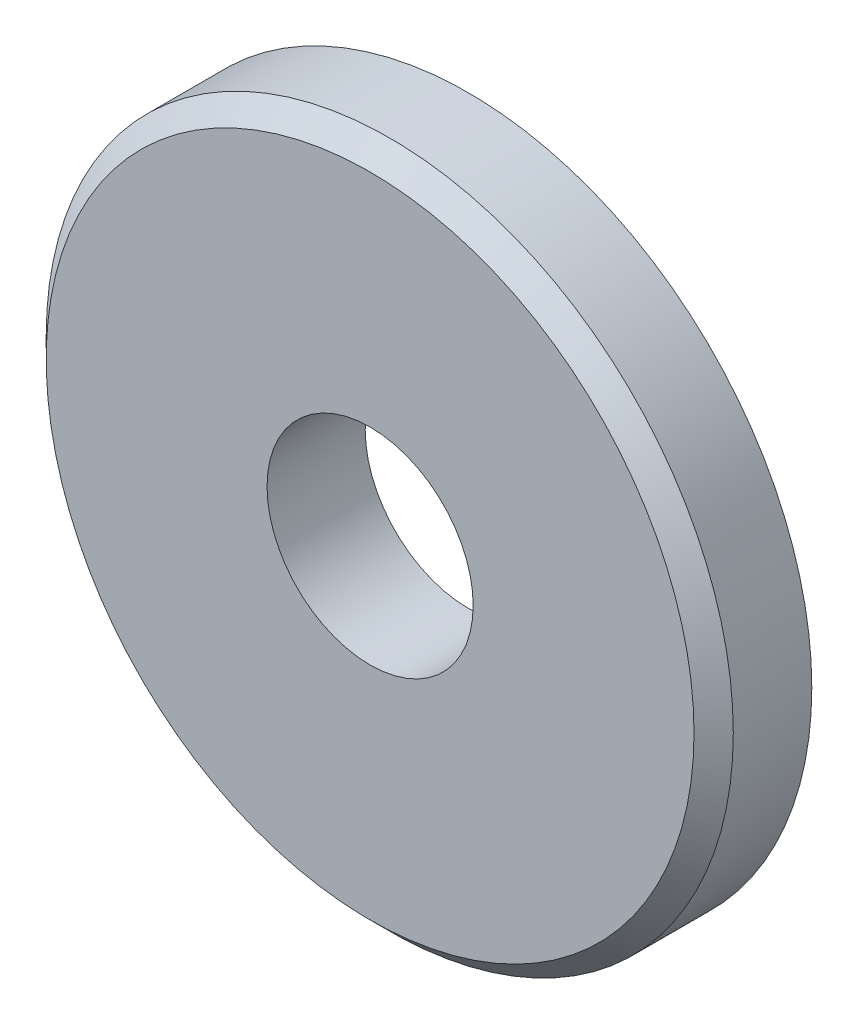
from build123d import *

# Parameters (mm, degrees)
SKETCH_1_R      = 17.5
SKETCH_1_R_2    = 5.25
EXTRUDE_1_DEPTH = 5
CHAMFER_1_SIZE  = 1


with BuildPart() as part:
    # 草图1 → 凸台-拉伸1 (new body)
    with BuildSketch(Plane.XY):
        Circle(SKETCH_1_R)
        Circle(SKETCH_1_R_2, mode=Mode.SUBTRACT)
    extrude(amount=EXTRUDE_1_DEPTH)

    # 倒角1
    chamfer_1_edges = [part.edges().sort_by_distance(p)[0] for p in [
        (-17.5, 0, 5),
    ]]
    chamfer(chamfer_1_edges, length=CHAMFER_1_SIZE)


solid = part.part
